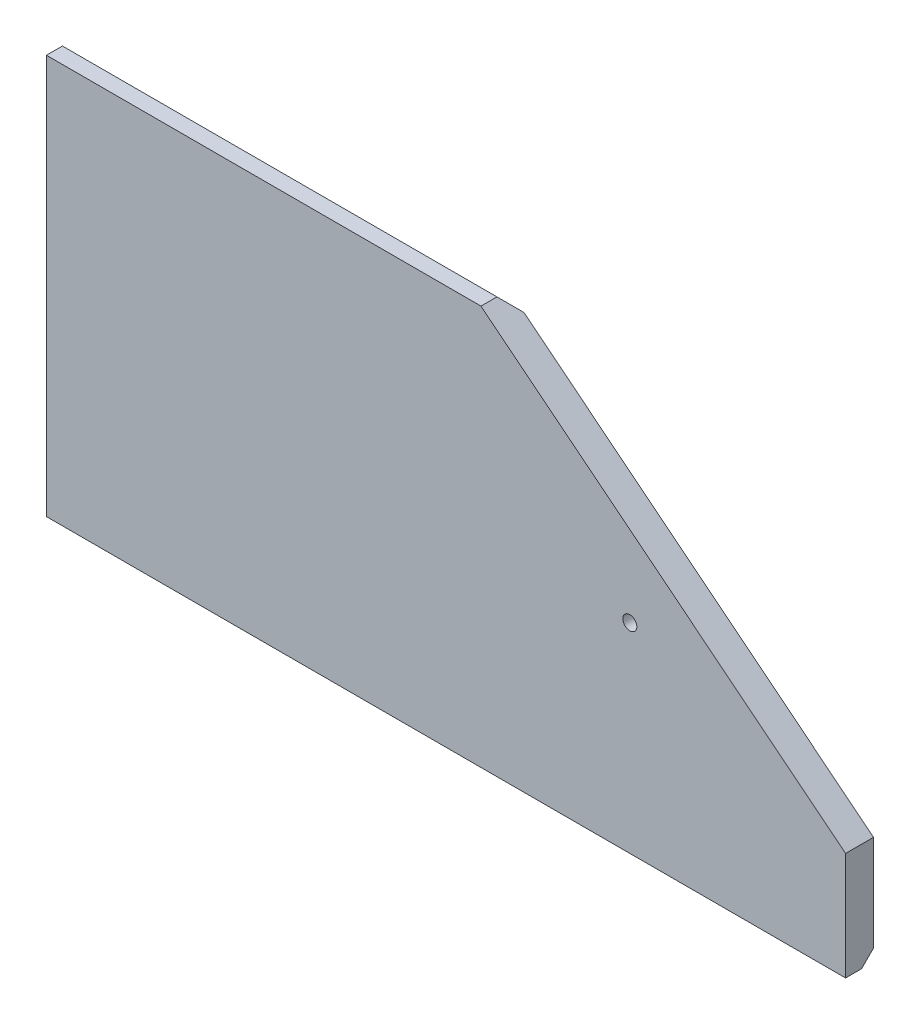
SolidWorks part; units mm, degrees
material "普通碳钢"
ref_plane "Front Plane" through (0, 0, 0) normal (0, 0, 1) x (1, 0, 0)
ref_plane "Top Plane" through (0, 0, 0) normal (0, 1, 0) x (1, 0, 0)
ref_plane "Right Plane" through (0, 0, 0) normal (1, 0, 0) x (0, 0, -1)
sketch "Sketch1" plane through (0, 0, 0) normal (0, 0, 1) x (1, 0, 0)
  line L1 (0, -25) -> (-1000, -25)
  line L2 (0, -25) -> (0, -525)
  line L3 (0, -525) -> (-1000, -525)
  line L4 (-1000, -25) -> (-1000, -525)
  dimension "D1" = 500
  dimension "D2" = 1000
extrude "Boss-Extrude1" add sketch "Sketch1" against normal blind 35
hole_wizard "M20 Tapped Hole1" positions "3DSketch1" profile "Sketch2" tap size "M20" standard "GB" end condition through all
sketch3d "3DSketch1"
  line L0 (0, -275, 0) -> (-1000, -275, 0) construction
  line L1 (0, -525, 0) -> (0, -25, 0) construction
  line L2 (-1000, -25, 0) -> (-1000, -525, 0) construction
  point P0 (-30, -275, 0)
  point P2 (-270, -275, 0)
  dimension "D1" = 30
  dimension "D2" = 240
sketch "Sketch2" plane through (-30, -275, 0) normal (1, 0, 0) x (0, -1, 0)
  line L0 (0, 0) -> (0, 35)
  line L1 (0, 35) -> (8.75, 35)
  line L2 (8.75, 35) -> (8.75, 0)
  line L5 (8.75, 0) -> (0, 0)
  line L11 (0, -6.35) -> (0, 107.95) construction
  dimension "通孔螺纹孔钻头直径" = 17.5
  dimension "通孔螺纹孔钻头深度" = 35
cosmetic thread "Tapped hole thread 1" parameters "D2"=20
cosmetic thread "Tapped hole thread 2" parameters "D2"=20
chamfer "Chamfer1" distance 15 angle 45 2 edges at (-500, -25, -35) (-500, -525, -35)
sketch "Sketch4" plane through (0, 0, 0) normal (0, 0, 1) x (1, 0, 0)
  line L4 (0, -525) -> (0, -25)
  line L6 (-1000, -25) -> (-1000, -525)
  line L10 (-1000, -25) -> (-1000, -525)
  line L14 (0, -25) -> (-1000, -25)
  line L15 (0, -25) -> (-1000, -25)
  line L16 (-1000, -525) -> (0, -525)
  line L17 (-1000, -525) -> (0, -525)
  dimension "D1" = 0
sketch "Sketch8" plane through (0, -525, 0) normal (0, -1, 0) x (1, 0, 0)
  line L0 (-500, 0) -> (0, 0)
  line L2 (0, 0) -> (0, -300)
  line L3 (0, -300) -> (-500, 0)
  dimension "D1" = 500
  dimension "D2" = 300
sketch "Sketch9" plane through (0, 0, 0) normal (0, 0, 1) x (1, 0, 0)
  line L0 (-500, 10) -> (0, 10)
  line L1 (0, -25) -> (-1000, -25) construction
  line L2 (0, 10) -> (0, -390)
  line L3 (0, -525) -> (0, -25) construction
  line L4 (0, -390) -> (-500, 10)
  dimension "D1" = 500
  dimension "D2" = 400
  dimension "D3" = 35
extrude "Cut-Extrude3" cut sketch "Sketch9" against normal through all
